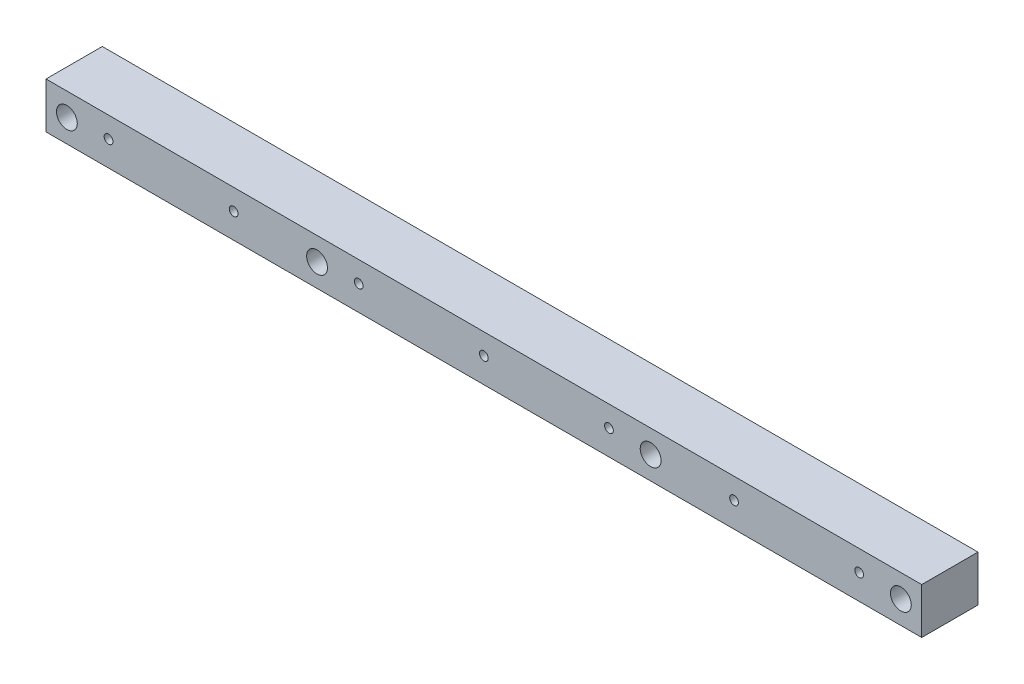
from build123d import *

# Parameters (mm, degrees)
SKETCH1_W                                           = 420
SKETCH1_H                                           = 22
BOSS_EXTRUDE1_DEPTH                                 = 27
M5_TAPPED_HOLE1_D                                   = 4.2
M5_TAPPED_HOLE1_DEPTH                               = 12.4
M5_TAPPED_HOLE1_TIP                                 = 1.2618073
CBORE_FOR_M5_HEX_SOCKET_HEAD_CAP_SCREW1_D           = 5.5
CBORE_FOR_M5_HEX_SOCKET_HEAD_CAP_SCREW1_CBORE_D     = 10
CBORE_FOR_M5_HEX_SOCKET_HEAD_CAP_SCREW1_CBORE_DEPTH = 17


with BuildPart() as part:
    # Sketch1 → Boss-Extrude1 (new body)
    with BuildSketch(Plane.XY):
        Rectangle(SKETCH1_W, SKETCH1_H)
    extrude(amount=BOSS_EXTRUDE1_DEPTH)

    # M5 Tapped Hole1
    with Locations(Plane.XY.offset(27)):
        with Locations((-180, 1), (-120, 1), (-60, 1), (0, 1), (60, 1), (120, 1), (180, 1)):
            Hole(M5_TAPPED_HOLE1_D / 2, depth=M5_TAPPED_HOLE1_DEPTH)
            with Locations((0, 0, -(M5_TAPPED_HOLE1_DEPTH + M5_TAPPED_HOLE1_TIP / 2))):  # 118° drill point
                Cone(0, M5_TAPPED_HOLE1_D / 2, M5_TAPPED_HOLE1_TIP, mode=Mode.SUBTRACT)

    # CBORE for M5 Hex Socket Head Cap Screw1 (through all)
    with Locations(Plane.XY.offset(27)):
        with Locations((-200, 0), (-80, 0), (80, 0), (200, 0)):
            CounterBoreHole(CBORE_FOR_M5_HEX_SOCKET_HEAD_CAP_SCREW1_D / 2, CBORE_FOR_M5_HEX_SOCKET_HEAD_CAP_SCREW1_CBORE_D / 2, CBORE_FOR_M5_HEX_SOCKET_HEAD_CAP_SCREW1_CBORE_DEPTH)


solid = part.part
